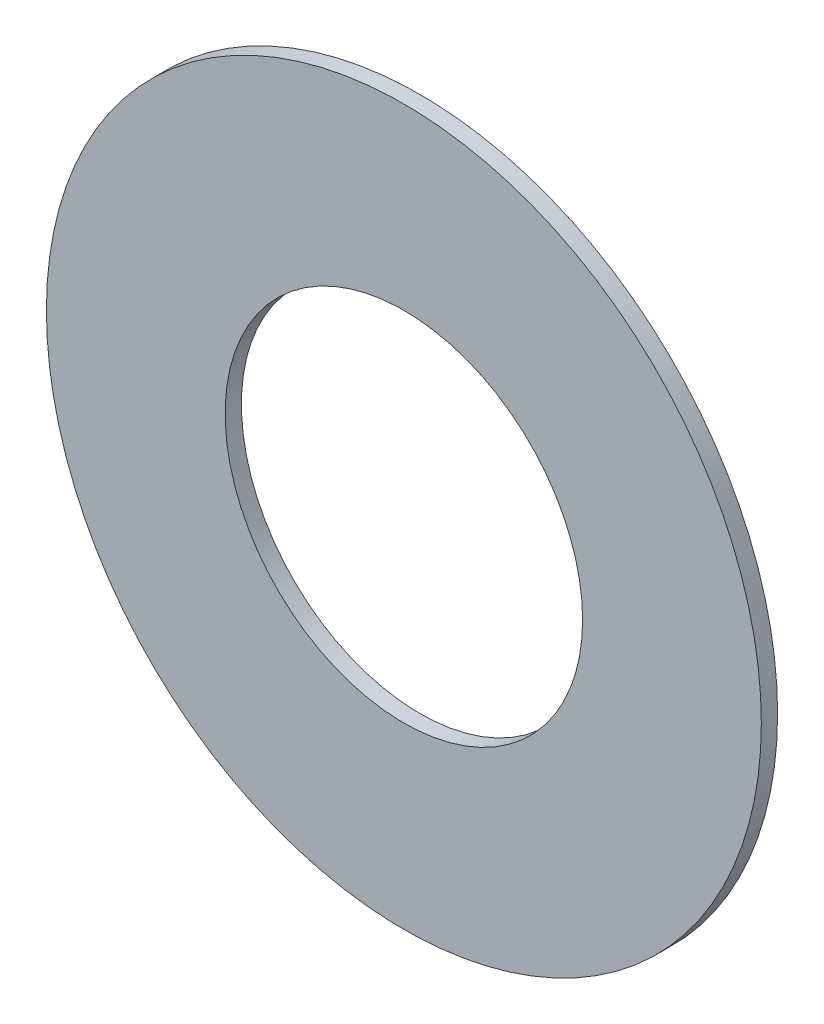
from build123d import *

# Parameters (mm, degrees)
SKETCH1_R           = 110
SKETCH1_R_2         = 55
BOSS_EXTRUDE3_DEPTH = 5


with BuildPart() as part:
    # Sketch1 → Boss-Extrude3 (new body)
    with BuildSketch(Plane.XY):
        with Locations((-2.7170484, 0.583803612)):
            Circle(SKETCH1_R)
        with Locations((-2.7170484, 0.583803612)):
            Circle(SKETCH1_R_2, mode=Mode.SUBTRACT)
    extrude(amount=BOSS_EXTRUDE3_DEPTH)


solid = part.part
